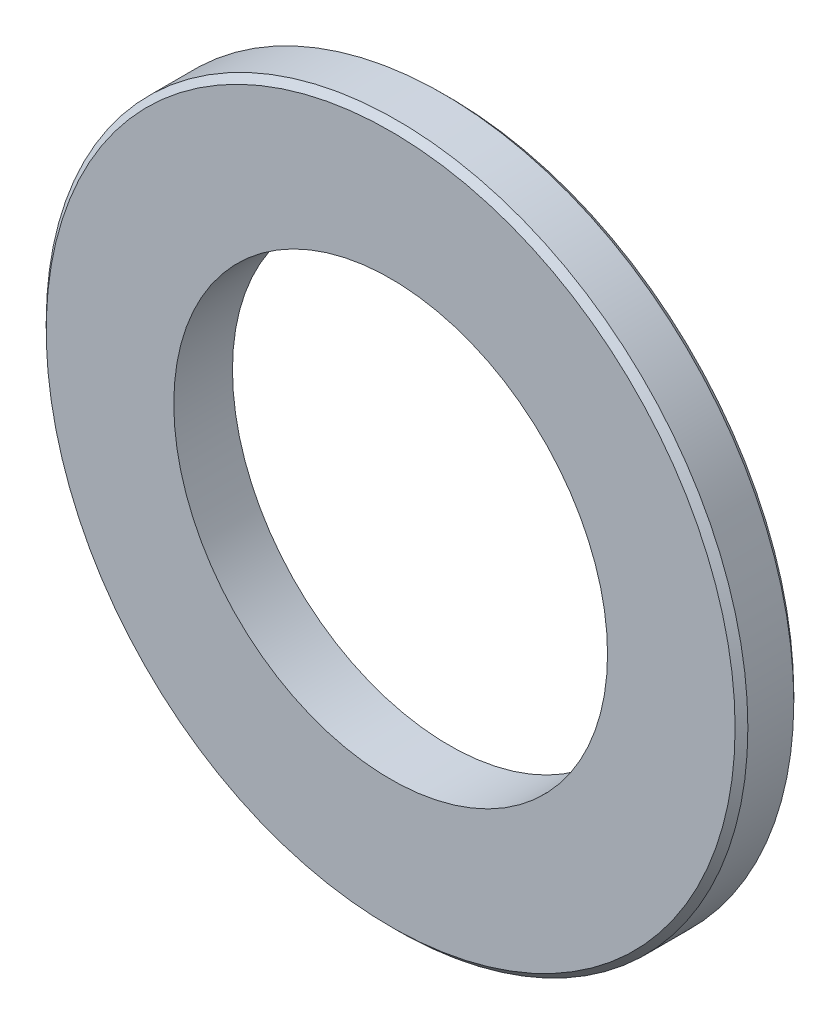
SolidWorks part; units mm, degrees
material "普通碳钢"
ref_plane "前视" through (0, 0, 0) normal (0, 0, 1) x (1, 0, 0)
ref_plane "上视" through (0, 0, 0) normal (0, 1, 0) x (1, 0, 0)
ref_plane "右视" through (0, 0, 0) normal (1, 0, 0) x (0, 0, -1)
sketch "草图1" plane through (0, 0, 0) normal (0, 0, 1) x (1, 0, 0)
  line L0 (-52.6001, 0) -> (57.3579, 0) construction
  line L1 (0, 38.1946) -> (0, -42.8202) construction
  circle A0 centre (0, 0) radius 27.5
  circle A1 centre (0, 0) radius 17
  dimension "D1" = 55
  dimension "D2" = 34
extrude "凸台-拉伸1" add sketch "草图1" along normal blind 4.6
chamfer "倒角1" distance 0.5 angle 45 2 edges at (27.5, 0, 0) (27.5, 0, 4.6)
